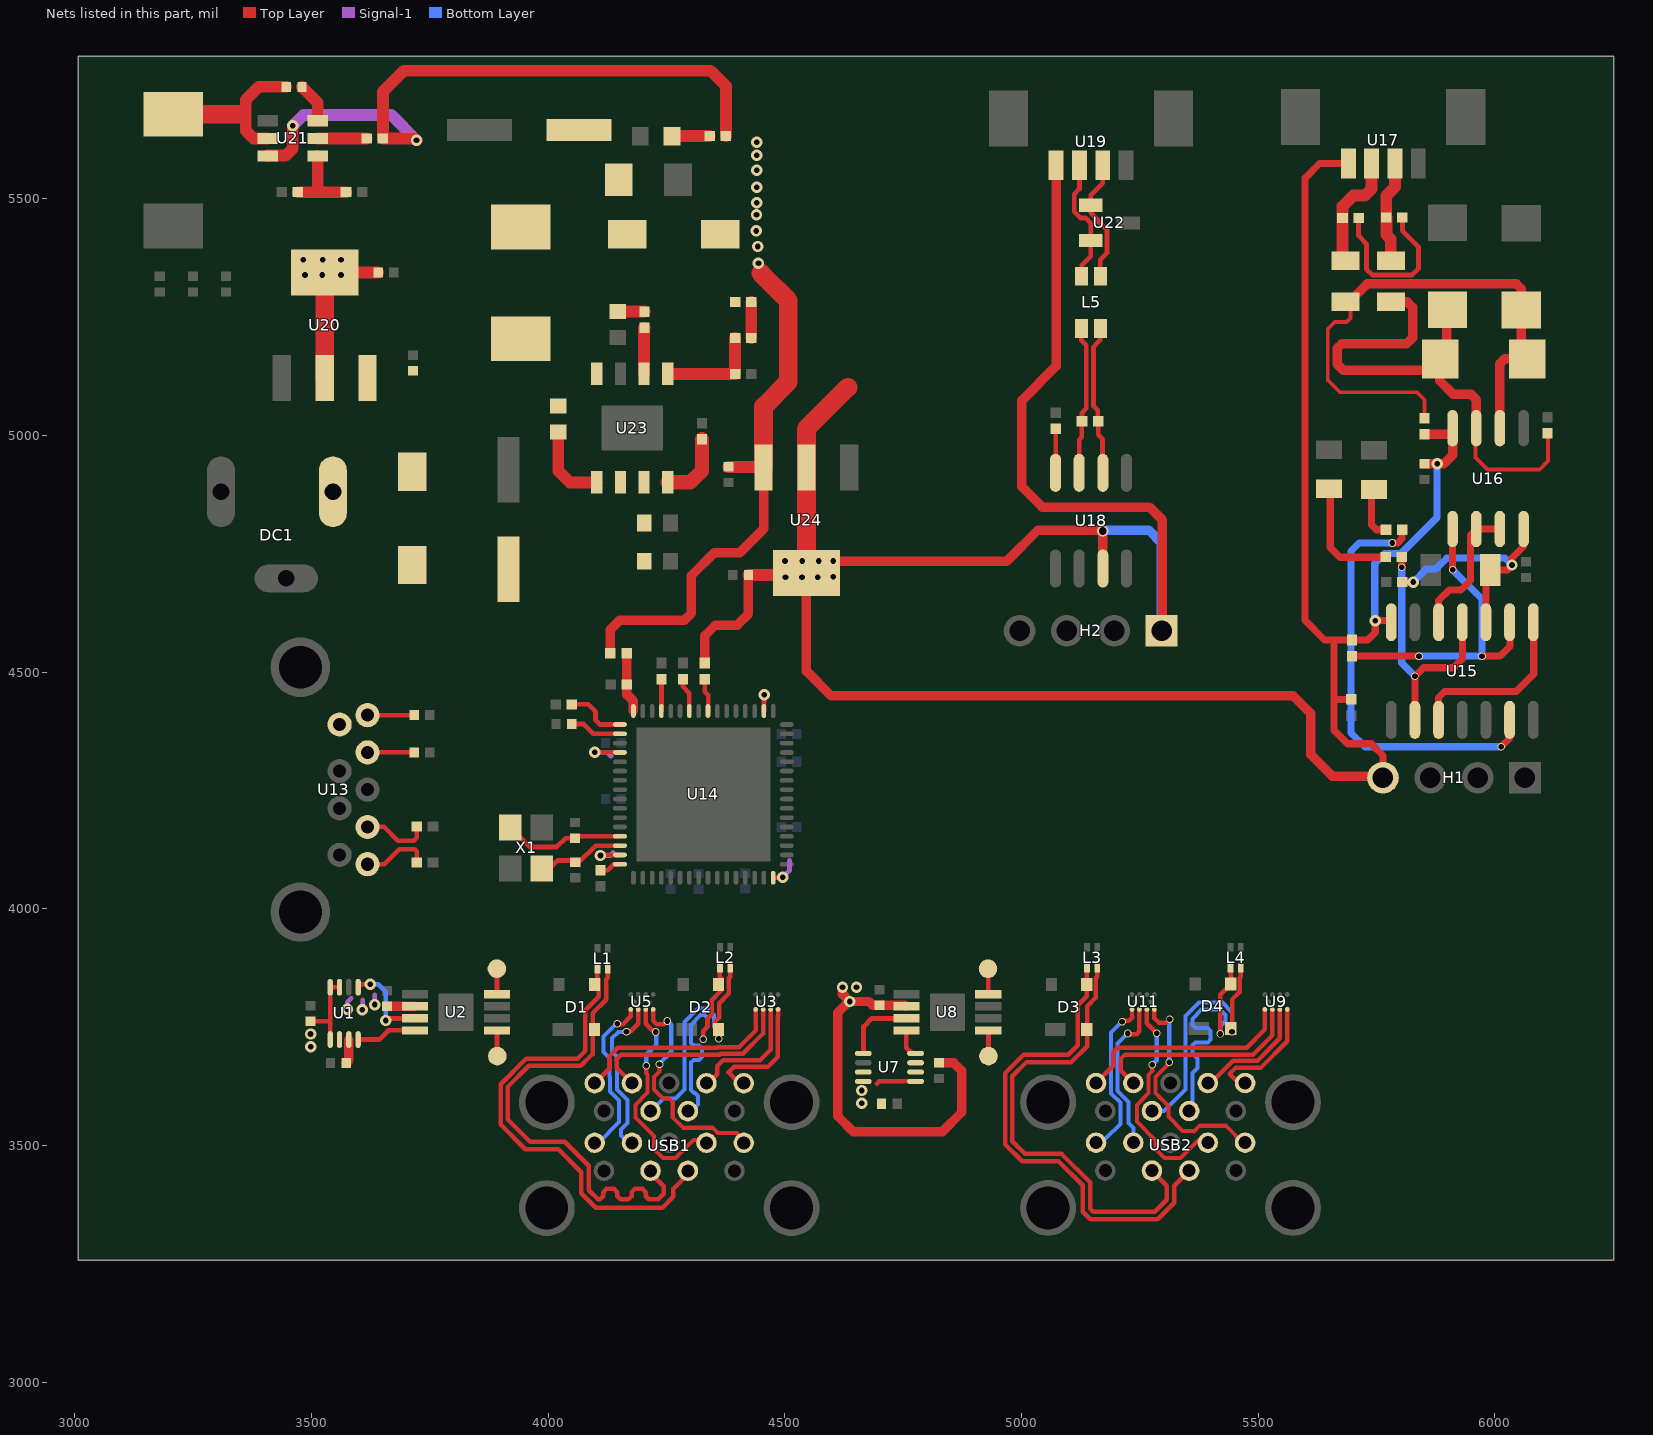
[diagram p0: the nets of this part, all layers, seen from the top]
# Altium PCB MISC51972.pcbdoc (part 2 of 3)
Units mil, origin at the board's own origin, x right, y up, seen from the top; angles counter-clockwise.
Board outline 3243 x 2543 mil, 4 copper layers (Top Layer, GND, Signal-1, Bottom Layer), stack 62.447 mil thick; 117 components, 123 nets, 473 pads, 324 vias.

## Via types
v1: diameter 24.02, hole 12, Top Layer to Bottom Layer, 276 vias
v2: diameter 16, hole 12, Top Layer to Bottom Layer, 47 vias
v3: diameter 24, hole 16, Top Layer to Bottom Layer, 1 vias

## Nets (pads, with @x,y where several pads share a name; then routed paths per layer and width w, separated by ;. In a path a pad name is that pad's centre, name@x,y a point inside that pad or via, vN(x,y) a via of type N, cw(c..) or ccw(c..) an arc to the next point about the centre after c; other vN are vias at no path point) (continued)
1.8V: C3.1 C6.1 C28.2 U1.3 U1.4 U1.5 U7.3 U7.4 U7.5 U20.2 U20.4 | length 591.4
  Top Layer w10: C3.1@3497.8,3762.76 3538.48,3762.76 3539.27,3761.97 ; U1.5@3539.27,3724.18 3539.27,3761.97 ; U1.3@3558.96,3834.62 U1.4@3539.27,3834.62 3539.27,3761.97 ; 4694.5,3631 4699.25,3635.75 U7.5@4775.99,3635.75
  Top Layer w25: U20.4@3527.7,5344.61 3640.35,5344.61 C28.2@3640.46,5344.5
  Top Layer w40: U20.2@3527.7,5121.39 U20.4@3527.7,5344.61
  other v1: 4662.5,3589.86 4662.5,3616.5 3498.5,3709 3497.8,3735.76 3485.87,5339.5 3522.76,5339.5 3562,5339.5 3482.5,5371.5 3523.5,5371.5 3561.93,5371.5
3.3V: C15.1 C36.2 H1.4 H2.1 R5.2 R6.2 R8.2 R14.2 U14.16 U14.34 U14.52 U14.63 U15.14 U16.8 U17.4 U18.3 U19.4 U24.2 U24.4 | length 7174.4
  Top Layer w10: v1@4098.5,4331.07 4151.02,4331.07 U14.52@4151.41,4330.68 ; v1@4110.15,4113.07 v1(4110.15,4112.92) 4111.38,4114.15 U14.63@4151.41,4114.15 ; U14.34@4455.54,4418.28 4455.54,4451.54 v1(4456.5,4452.5) ; U14.16@4475.23,4065.92 4494.42,4065.92 v1(4495.5,4067)
  Top Layer w15: U17.4@5690.33,5574.64 5629.64,5574.64 5599.1,5544.1 5599.1,4609.1 5640,4568.2 5659.6,4568.2 ; R5.2@5696.45,4442.7 5659.6,4442.7 ; H1.4@5763.5,4277.5 5763.5,4324.2 5738.6,4349.1 5688.6,4349.1 5659.6,4378.1 5659.6,4442.7 ; U15.14@5780.95,4605.77 5777.62,4609.1 v1(5747.1,4609.1) 5747.1,4584.1 5731.6,4568.6 5698.85,4568.6 R6.2@5698.45,4568.2 5659.6,4568.2 ; 5659.6,4442.7 5659.6,4568.2
  Top Layer w20: R14.2@4330.6,4519.64 4330.6,4577.36 4352.74,4599.5 4399,4599.5 4422.84,4623.34 C36.2@4422.84,4705.5 ; U24.4@4545.4,4709.29 4545.4,4502.6 4598,4450 5574,4450 5611,4413 5611,4326 5656.5,4280.5 5760.5,4280.5 H1.4@5763.5,4277.5 ; v1(4602.04,4735) 4969,4735 5034,4800 5170.14,4800 v3(5171.64,4798.5) U18.3@5171.64,4719.18 ; U19.4@5073.02,5571.14 5073.02,5147.02 5000.5,5074.5 5000.5,4892 5043.5,4849 5270,4849 5297.5,4821.5 5297.5,4589.71 H2.1@5295.64,4587.86 ; C15.1@5851,4940.54 v1(5878,4940.54) 5892.04,4940.54 5911.1,4959.6 5911.1,5015.01 U16.8@5910.45,5015.66 5910.45,5002.46 R8.2@5851,5002.46
  Top Layer w25: C36.2@4422.84,4705.5 4541.61,4705.5 U24.4@4545.4,4709.29
  Top Layer w40: U24.4@4545.4,4709.29 U24.2@4545.4,4932.51 4545.4,5014.4 4633,5102
  Signal-1 w10: v1(4098.5,4330.89) 4124.61,4330.89 4132.5,4323 ; v1(4110.15,4112.92) 4130.92,4112.92 4137.5,4119.5 ; v1(4495.5,4067) 4509.5,4081 4509.5,4103
  Bottom Layer w15: v1(5747.1,4609.1) 5746.1,4610.1 5746.1,4730.1 5766.6,4750.6 5801.1,4750.6 5878,4827.5 v1(5878,4940.54)
  Bottom Layer w20: v3(5171.64,4798.5) 5173.14,4800 5269,4800 5295.5,4773.5 5295.5,4588 H2.1@5295.64,4587.86
  other v1: 4501,4701 4536.05,4701 4569.5,4701 4602.04,4702.08 4500,4735 4536.48,4735 4571.39,4735
12V: C27.2 D10.1 DC1.1 U20.3
485-1: U15.12 U16.2 U16.3 | length 294.2
  Top Layer w15: U15.12@5880.95,4605.77 5880.95,4651.45 5903.6,4674.1 5928.1,4674.1 5948.1,4694.1 5948.1,4790.31 U16.2@5960.45,4802.66 U16.3@6010.45,4802.66
485-7: D6.1 D7.2 F2.1 R16.2 U16.7 | length 1151.4
  Top Layer w8: U16.7@5960.45,5015.66 5958.95,5014.16 5958.95,4953.75 5984.2,4928.5 6094.5,4928.5 6112.1,4946.1 6112.1,5003.93 R16.2@6111.45,5004.58
  Top Layer w20: F2.1@5779.95,5282.86 5814.34,5282.86 5826.1,5271.1 5826.1,5206.6 5813.5,5194 5676.5,5194 5666.6,5184.1 5666.6,5151.1 5679.1,5138.6 5861.37,5138.6 D6.1@5883.27,5160.5 ; D7.2@5899.45,5265.93 5897.95,5264.43 5897.95,5175.18 D6.1@5884.77,5162 D6.1@5883.27,5160.5 ; U16.7@5960.45,5015.66 5960.45,5076.25 5949.7,5087 5912.2,5087 5883.27,5115.93 D6.1@5883.27,5160.5
$1N3773: U1.8 U2.4 | length 128.3
  Top Layer w10: U1.8@3598.33,3724.18 3643.18,3724.18 3662.5,3743.5 3718.2,3743.5 U2.4@3718.49,3743.21
$1N3774: U1.1 U2.3 | length 192.1
  Top Layer w10: U1.1@3598.33,3834.62 3604.71,3841 v1(3624,3841) ; v1(3656.5,3764.41) 3660.89,3768.8 U2.3@3718.49,3768.8
  Bottom Layer w10: v1(3624,3841) 3641,3841 3656.5,3825.5 v1(3656.5,3764.41)
$1N3787: U7.8 U8.4 | length 60.9
  Top Layer w10: U8.4@4756.39,3743.21 4756.39,3707 4768.58,3694.81 U7.8@4775.99,3694.81
$1N3788: U7.1 U8.3 | length 154.4
  Top Layer w10: U7.1@4665.55,3694.81 4666,3695.26 4666,3751.5 4683.3,3768.8 U8.3@4756.39,3768.8
$1N3806: D1.2 L1.2 USB1.2 | length 1020.7
  Top Layer w9.5: L1.2@4125.43,3873.15 4125.43,3854.5 4122.35,3851.42 4122.35,3808.43 4093.46,3779.54 4093.46,3693.58 4068.38,3668.5 3958.51,3668.5 3914,3623.99 3914,3555.5 3961.5,3508 4034.5,3508 4085.31,3457.19 4085.31,3433.43 4085.5,3433.24 4085.5,3406 4105,3386.5 4109.17,3386.5 4115.89,3393.22 4115.89,3401.71 4122.6,3408.42 4139.17,3408.42 4145.89,3401.71 4145.89,3393.22 4152.6,3386.5 4169.17,3386.5 4175.89,3393.22 4175.89,3401.78 4182.6,3408.5 4199.17,3408.5 4205.89,3401.78 4205.89,3393.22 4212.6,3386.5 4232.35,3386.5 4244.04,3398.19 4244.04,3414.11 4217.43,3440.73 USB1.2@4217.43,3447.15
$1N3807: D1.3 L1.3 USB1.3 | length 1020.7
  Top Layer w9.5: L1.3@4103.77,3873.15 4103.77,3854.5 4106.85,3851.42 4106.85,3814.85 4077.96,3785.96 4077.96,3700 4061.96,3684 3953.5,3684 3899.5,3630 3899.5,3544.5 3951.5,3492.5 4021.5,3492.5 4070,3444 4070,3399.58 4100.58,3369 4241.32,3369 4264,3391.68 4264,3408.5 4296.17,3440.67 USB1.3@4296.17,3447.15
$1N3813: D2.3 L2.3 USB1.12 | length 496.7
  Top Layer w9.5: v2(4327.28,3724.72) 4327.28,3742.22 4335.89,3750.83 4335.89,3767.53 4345.46,3777.1 4345.46,3807.46 4365.75,3827.75 4365.75,3853.42 4362.67,3856.5 L2.3@4362.67,3875.15
  Bottom Layer w8.5: USB1.12@4294.86,3572.83 4299.03,3572.83 4307.39,3581.19 4309.83,3581.19 4315.84,3587.2 4315.84,3605.18 4309.83,3611.19 4307.39,3611.19 4301.38,3617.2 4301.38,3675.18 4307.39,3681.19 4318.48,3681.19 4324.49,3687.2 4324.49,3705.18 4318.48,3711.19 4307.39,3711.19 4301.38,3717.2 4301.38,3755.12 4321.88,3775.62 4330.38,3775.62 4336.39,3769.61 4336.39,3750.33 4327.28,3741.22 v2(4327.28,3724.72)
$1N3814: D2.2 L2.2 USB1.11 | length 537.9
  Top Layer w9.5: D2.2@4359.8,3745.56 4360,3745.36 D2.2@4360,3743 ; v2(4360,3725.5) D2.2@4360,3743 ; L2.2@4384.33,3875.15 4384.33,3856.5 4381.25,3853.42 4381.25,3821.33 4360.96,3801.04 4360.96,3770.68 4351.39,3761.11 4351.39,3751.61 D2.2@4360,3743
  Bottom Layer w8.5: USB1.11@4216.12,3572.83 4243.3,3600 4268.7,3600 4287.38,3618.68 4287.38,3761.63 4315.88,3790.12 4336.39,3790.12 4350.5,3776.01 4350.5,3751.5 4360,3742 v2(4360,3725.5)
$1N3821: D3.2 L3.2 USB2.2 | length 1001.1
  Top Layer w9.5: L3.2@5159.83,3875.15 5159.83,3856.5 5156.75,3853.42 5156.75,3812.83 5138.46,3794.54 5138.46,3710.04 5104.92,3676.5 5010.42,3676.5 4980.46,3646.54 4980.46,3509.46 5007.46,3482.46 5084.46,3482.46 5144.5,3422.42 5144.5,3367 5151.22,3360.28 5281.5,3360.28 5306.92,3385.71 5306.92,3415.53 USB2.2@5275.3,3447.15
$1N3822: D3.3 L3.3 USB2.3 | length 1049.9
  Top Layer w9.5: L3.3@5138.17,3875.15 5137.5,3874.48 5137.5,3815.5 5118.86,3796.86 5118.86,3712.36 5098.5,3692 5004,3692 4964.96,3652.96 4964.96,3503.04 5001.04,3466.96 5078.04,3466.96 5129,3416 5129,3360.58 5144.8,3344.78 5287.92,3344.78 5322.42,3379.29 5322.42,3415.53 USB2.3@5354.04,3447.15
$1N3827: D4.3 L4.3 USB2.12 | length 547.3
  Top Layer w9.5: v2(5419.76,3736) 5419.76,3819.03 5444.65,3843.92 5444.65,3853.42 5441.57,3856.5 L4.3@5441.57,3875.15
  Bottom Layer w8.5: USB2.12@5354.04,3573.13 5361,3580.09 5361,3653.56 5371.82,3664.38 5371.82,3683.56 5361,3694.38 5361,3712.36 5367.01,3718.37 5393.25,3718.37 5399.26,3724.38 5399.26,3742.36 5393.25,3748.37 5367.01,3748.37 5361,3754.38 5361,3768 5380.5,3787.5 5419.41,3787.5 5431,3775.91 5431,3763.74 5419.76,3752.5 v2(5419.76,3736)
$1N3831: D4.2 L4.2 USB2.11 | length 546.7
  Top Layer w9.5: v2(5444.5,3740.5) 5444.5,3808.8 5460.55,3824.85 5460.55,3853.81 5463.23,3856.5 L4.2@5463.23,3875.15
  Bottom Layer w8.5: USB2.11@5275.3,3573.13 5300.71,3573.13 5346.56,3618.98 5346.56,3774.07 5374.49,3802 5424.01,3802 5444.5,3781.51 v2(5444.5,3740.5)
$1N3840: U3.C1 USB1.18 | length 447.2
  Top Layer w9.5: USB1.18@4098.02,3631.89 4129.64,3663.51 4129.64,3678.35 cw(c4143.96,3680.61) 4129.5,3679.57 4128.46,3680.61 4128.46,3688.46 4147,3707 4357.02,3707 4358.31,3708.29 4403.29,3708.29 4438.26,3743.26 4438.26,3773.14 4438.13,3773.26 U3.C1@4438.13,3787.76
$1N3841: U3.C2 USB1.17 | length 447.2
  Top Layer w9.5: USB1.17@4176.76,3631.89 4145.14,3663.51 4145.14,3679.43 4143.96,3680.61 4143.96,3682.04 4153.42,3691.5 4362.03,3691.5 4364.32,3693.79 4410.71,3693.79 4453.76,3736.83 4453.76,3773.14 4453.88,3773.26 U3.C2@4453.88,3787.76
$1N3842: U3.C3 USB1.15 | length 260.1
  Top Layer w9.5: USB1.15@4334.23,3631.89 4338.39,3631.89 4357,3650.5 4357,3668.09 4369.7,3680.79 4447.71,3680.79 4469.62,3702.71 U3.C3@4469.62,3787.76
$1N3843: U3.C4 USB1.14 | length 260
  Top Layer w9.5: USB1.14@4412.98,3631.89 4403.61,3631.89 4380.61,3654.89 4392.01,3666.29 4463.46,3666.29 4485.24,3688.08 4485.24,3773.14 4485.37,3773.26 U3.C4@4485.37,3787.76
$1N3853: U9.C1 USB2.18 | length 463
  Top Layer w9.5: USB2.18@5157.19,3632.19 5193.46,3668.46 5193.46,3697.46 5203,3707 5475.49,3707 5514.08,3745.59 U9.C1@5514.08,3787.76
$1N3854: U9.C2 USB2.17 | length 458.4
  Top Layer w9.5: USB2.17@5235.93,3632.19 5208.96,3659.16 5208.96,3683 5218.46,3692.5 5489.5,3692.5 5529.7,3732.7 5529.7,3773.14 5529.83,3773.26 U9.C2@5529.83,3787.76
$1N3855: U9.C3 USB2.15 | length 252.4
  Top Layer w9.5: USB2.15@5393.41,3632.19 5399.46,3632.19 5446.77,3679.5 5498.19,3679.5 5545.69,3727 5545.69,3773.14 5545.57,3773.26 U9.C3@5545.57,3787.76
$1N3856: U9.C4 USB2.14 | length 258.4
  Top Layer w9.5: USB2.14@5472.15,3632.19 5458.81,3632.19 5439.39,3651.61 5452.78,3665 5505.62,3665 5561.19,3720.58 5561.19,3773.14 5561.32,3773.26 U9.C4@5561.32,3787.76
$1N3865: U5.C4 USB1.5 | length 481.2
  Top Layer w8.5: v2(4235,3672) 4235,3656.49 4223.61,3645.1 4223.61,3618.68 4242.29,3600 4255.5,3600 4262.98,3592.52 4262.98,3559.62 4284.81,3537.79 4347.44,3537.79 4358.82,3526.41 4398.47,3526.41 4412.98,3511.91 USB1.5@4412.98,3505.9
  Top Layer w9.5: U5.C4@4221.62,3787.76 4221.62,3773.26 4221.49,3773.14 4221.49,3763.64 4228.21,3756.92 4245,3756.92 v2@4251.34,3763.26
  Bottom Layer w9.5: v2(4235,3672) 4235,3673.5 4259.5,3698 4259.5,3755.2 v2(4251.34,3763.36)
$1N3866: U5.C3 USB1.6 | length 480.7
  Top Layer w8.5: v2(4207,3669) 4207,3652.5 4210.11,3649.39 4210.11,3611.91 4184.24,3586.04 4184.24,3559.62 4223.61,3520.25 4223.61,3492.69 4242.29,3474.01 4268.7,3474.01 4306.6,3511.91 4328.23,3511.91 USB1.6@4334.23,3505.9
  Top Layer w9.5: U5.C3@4205.87,3787.76 4205.87,3773.26 4205.99,3773.14 4205.99,3757.22 4221.79,3741.42 4225.96,3741.42 v2(4227.34,3740.04)
  Bottom Layer w9.5: v2(4207,3669) 4207,3692 4228.5,3713.5 4228.5,3738.88 v2(4227.34,3740.04)
$1N3867: U5.C2 USB1.8 | length 352.3
  Top Layer w9.5: v2(4165.28,3740.55) 4173.05,3740.55 4190.01,3757.51 4190.01,3773.5 4190.13,3773.62 U5.C2@4190.13,3787.76
  Bottom Layer w8.5: v2(4165.28,3740.55) 4148.05,3740.55 4134.99,3727.49 4134.99,3698.4 4144.87,3688.52 4144.87,3618.68 4167,3596.55 4167,3548 4153.5,3534.5 4153.5,3521.5 4169.1,3505.9 USB1.8@4176.76,3505.9
$1N3868: U5.C1 USB1.9 | length 354.9
  Top Layer w9.5: v2(4146.02,3757.35) 4147.65,3757.35 4148.25,3756.75 4157.75,3756.75 4174.51,3773.5 4174.38,3773.62 U5.C1@4174.38,3787.76
  Bottom Layer w8.5: USB1.9@4098.02,3505.9 4105.81,3505.9 4149.58,3549.68 4149.58,3594.92 4129.9,3614.6 4129.9,3645.1 4129,3646 4129,3685.3 4116.5,3697.8 4116.5,3730.5 4143.35,3757.35 v2(4146.02,3757.35)
$1N3877: U11.C4 USB2.5 | length 482
  Top Layer w8.5: 5282.55,3618.74 5282.79,3618.5 ; v2(5312.12,3675.85) 5312.12,3674.74 5282.79,3645.4 5282.79,3618.5 ; USB2.5@5472.15,3506.2 5467.16,3506.2 5431.36,3542 5376.11,3542 5364.1,3529.99 5362.86,3531.24 5339.84,3531.24 5310,3561.08 5310,3584.1 5282.79,3611.31 5282.79,3618.5
  Top Layer w9.5: U11.C4@5280.47,3787.76 5280.47,3769.53 5290.25,3759.75 5305.5,3759.75 v2(5312.62,3766.88)
  Bottom Layer w9.5: v2(5312.12,3675.85) 5312.12,3766.38 v2(5312.62,3766.88)
$1N3878: U11.C3 USB2.6 | length 473.7
  Top Layer w8.5: v2(5276,3670.85) 5276,3657.7 5267.82,3649.52 5267.82,3610.74 5243.42,3586.34 5243.42,3550.58 5282.79,3511.21 5282.79,3492.99 5301.47,3474.31 5336.11,3474.31 5374.01,3512.21 5387.4,3512.21 USB2.6@5393.41,3506.2
  Top Layer w9.5: U11.C3@5264.72,3787.76 5264.72,3758.28 v2(5285.5,3737.5)
  Bottom Layer w9.5: v2(5276,3670.85) 5285.5,3680.35 v2(5285.5,3737.5)
$1N3879: U11.C2 USB2.8 | length 327.7
  Top Layer w9.5: v2(5224.41,3736.82) 5225.74,3735.5 5243,3735.5 5248.85,3741.36 5248.85,3773.14 5248.98,3773.26 U11.C2@5248.98,3787.76
  Bottom Layer w8.5: v2(5224.41,3736.82) 5223.82,3736.82 5202.58,3715.58 5202.58,3615.92 5226,3592.51 5226,3547.5 5235.93,3537.57 USB2.8@5235.93,3506.2
$1N3880: U11.C1 USB2.9 | length 343.8
  Top Layer w9.5: v2(5212.28,3761.81) 5214.11,3763.64 5226.64,3763.64 5233.35,3770.35 5233.35,3773.14 5233.23,3773.26 U11.C1@5233.23,3787.76
  Bottom Layer w8.5: USB2.9@5157.19,3506.2 5165.69,3514.7 5177.71,3514.7 5208.76,3545.75 5208.76,3590.65 5189.08,3610.33 5189.08,3738.61 v2(5212.28,3761.81)
$1N5034: C9.2 U14.62 X1.1 | length 187.8
  Top Layer w10: X1.1@3986.47,4085.89 4003.39,4085.89 4020,4102.5 4053.34,4102.5 C9.2@4057,4098.84 4064.84,4098.84 4099.83,4133.83 U14.62@4151.41,4133.83
$1N5035: C10.2 U14.61 X1.3 | length 258.4
  Top Layer w10: X1.3@3919.53,4172.51 3961.05,4131 4018,4131 4036.56,4149.56 C10.2@4056.7,4149.56 4060.66,4153.52 U14.61@4151.41,4153.52
$1N5041: R3.1 U14.64 | length 46.6
  Top Layer w10: R3.1@4110,4082.04 4125.54,4082.04 4137.96,4094.46 U14.64@4151.41,4094.46
$1N5046: C17.1 U14.50 | length 110.6
  Top Layer w10: C17.1@4049.34,4390.72 4074.78,4390.72 4095.45,4370.05 U14.50@4151.41,4370.05
$1N5048: R11.1 U14.49 | length 129.5
  Top Layer w10: R11.1@4049.84,4432.4 4084.1,4432.4 4100,4416.5 4100,4399 4109.26,4389.74 U14.49@4151.41,4389.74
$1N5050: R7.1 R9.1 U14.48 | length 128.1
  Top Layer w20: R7.1@4165.33,4540.28 4165.33,4474.77 R9.1@4166.2,4473.9 4166.2,4452.8 4179.95,4439.05 U14.48@4179.95,4418.28
$1N5101: R12.1 U14.45 | length 67.3
  Top Layer w10: U14.45@4239.01,4418.28 4239.1,4418.37 R12.1@4239.1,4485.56
$1N5103: R13.1 U14.42 | length 72.7
  Top Layer w10: R13.1@4284.8,4485.56 4284.8,4469.2 4298,4456 U14.42@4298,4418.34
$1N5105: R14.1 U14.40 | length 70.6
  Top Layer w10: R14.1@4330.6,4485.56 4330.6,4458.9 4338,4451.5 4338,4418.85 U14.40@4337.43,4418.28
$1N8075: R6.1 U15.9 U16.1 | length 687.8
  Top Layer w15: R6.1@5698.45,4534.12 v2(5839.6,4534.1) ; U16.1@5910.45,4802.66 5910.6,4802.51 v2(5910.6,4716.6) ; v2(5972.6,4534.1) 6011.1,4534.1 6032.1,4555.1 6032.1,4604.62 U15.9@6030.95,4605.77
  Bottom Layer w15: v2(5839.6,4534.1) v2(5972.6,4534.1) 5972.6,4654.6 v2(5910.6,4716.6)
$1N8076: R17.1 U15.2 U15.11 | length 548.7
  Top Layer w15: v2(5803.1,4722.1) 5803.1,4742.77 R17.1@5803.49,4743.16 ; U15.2@5830.95,4399.55 v2(5830.95,4491.6) 5848.95,4509.6 5912.6,4509.6 5931.6,4528.6 5931.6,4605.12 U15.11@5930.95,4605.77
  Bottom Layer w15: v2(5803.1,4722.1) 5803.1,4519.45 v2(5830.95,4491.6)
$1N8077: R18.2 U15.6 | length 915
  Top Layer w15: v2(5783.1,4773.1) 5794.6,4773.1 5803.95,4782.45 R18.2@5803.95,4801.16 ; v2(6013.1,4342.6) 6030.95,4360.45 U15.6@6030.95,4399.55
  Bottom Layer w15: v2(5783.1,4773.1) 5713.1,4773.1 5696.1,4756.1 5696.1,4372.1 5725.6,4342.6 v2(6013.1,4342.6)
$1N8081: U15.3 U15.8 | length 378.8
  Top Layer w15: U15.3@5880.95,4399.55 5880.95,4446.45 5893.6,4459.1 6045.1,4459.1 6082.1,4496.1 6082.1,4604.62 U15.8@6080.95,4605.77
$1N8120: R4.2 R10.2 | length 358
  Top Layer w10: R4.2@5711.99,5460.16 5711.99,5422.01 5728.5,5405.5 5728.5,5352 5741,5339.5 5825,5339.5 5838.5,5353 5838.5,5399 5804.49,5433.01 R10.2@5804.49,5461.16
$1N8121: F2.2 R10.1 U17.2 | length 216.7
  Top Layer w25: F2.2@5779.95,5369.47 5779.95,5415.25 5770.6,5424.6 5770.6,5460.97 R10.1@5770.41,5461.16 5770.41,5506.91 5788.76,5525.26 U17.2@5788.76,5574.64
$1N8129: D5.1 D6.2 F1.1 R8.1 U16.6 | length 1189.9
  Top Layer w8: F1.1@5684.45,5282.86 5694.6,5272.71 5694.6,5248.1 5686.6,5240.1 5661.6,5240.1 5646.6,5225.1 5646.6,5117.6 5672.6,5091.6 5835.1,5091.6 5851,5075.7 R8.1@5851,5036.54
  Top Layer w20: F1.1@5684.45,5282.86 5692.36,5282.86 5730.5,5321 6044.7,5321 6055.45,5310.25 D5.1@6055.45,5265.43 6055.45,5162 6020.5,5162 6010.45,5151.95 U16.6@6010.45,5015.66
$1N8138: R17.2 TXD1.1 | length 251.1
  Top Layer w15: TXD1.1@5649.45,4887.82 5652.1,4885.17 5652.1,4763.6 5672.54,4743.16 R17.2@5769.41,4743.16
$1N8140: R18.1 RXD1.1 | length 112
  Top Layer w15: RXD1.1@5744.45,4886.32 5739.1,4880.97 5739.1,4811.6 5749.54,4801.16 R18.1@5769.87,4801.16
$1N8159: L5.4 R22.2 U18.7 | length 315.6
  Top Layer w10: U18.7@5121.64,4921.54 5121.64,4991.14 5127,4996.5 5127,5029.75 R22.2@5127.6,5030.36 5127.6,5048.6 5136.5,5057.5 5136.5,5190.5 5126,5201 5126,5225.28 L5.4@5126.96,5226.24
$1N8164: L5.1 R22.1 U18.6 | length 318.8
  Top Layer w10: L5.1@5166.33,5226.24 5166.33,5202.33 5152,5188 5152,5062.5 5161,5053.5 5161,5031.04 R22.1@5161.68,5030.36 5161.68,5001.82 5171,4992.5 5171,4922.18 U18.6@5171.64,4921.54
$1N8180: R19.1 U18.8 | length 93
  Top Layer w10: U18.8@5071.64,4921.54 5071.64,4950.54 5072.14,4951.04 R19.1@5072.14,5014.36
$1N8697: C7.1 U13.9 | length 98.7
  Top Layer w9.5: U13.9@3618.12,4409.47 3618.34,4409.68 C7.1@3716.71,4409.68
$1N8703: C8.1 U13.8 | length 98.5
  Top Layer w9.5: U13.8@3618.18,4330.78 C8.1@3716.71,4330.78
$1N8823: R1.1 U13.6 | length 142.8
  Top Layer w9.5: U13.6@3618.12,4173.25 3653.21,4173.24 3682.32,4144.13 3715.7,4144.13 3722.41,4150.85 R1.1@3722.41,4174.48
$1N8893: R2.1 U13.5 | length 142.8
  Top Layer w9.5: U13.5@3618.12,4094.51 3653.21,4094.5 3684.83,4126.12 3718.21,4126.12 3722.41,4121.92 R2.1@3722.41,4098.28
$1N10185: R24.2 R26.1 | length 76.2
  Top Layer w25: R26.1@4428.74,5206.35 R24.2@4428.74,5282.6
$1N10186: C30.2 C31.1 D9.1 L7.2
$1N10189: LED1.1 R25.2 | length 79.7
  Top Layer w25: LED1.1@4261.47,5632.7 R25.2@4341.16,5632.7
$1N10190: C37.1 R29.2 | length 56
  Top Layer w25: C37.1@4147.02,5262.04 R29.2@4203,5262.04
$1N10191: C29.2 U23.1 | length 173.7
  Top Layer w25: C29.2@4021.1,5007.6 4021.1,4925.4 4045.5,4901 4101.9,4901 U23.1@4102.3,4901.4
$1N10192: C32.1 C33.2 C34.2 D10.2 U23.2 U23.3
$1N10193: R27.2 U23.4 | length 148.7
  Top Layer w30: U23.4@4252.3,4901.4 4299.9,4901.4 4324.5,4926 R27.2@4324.5,4992.32
$1N10194: C29.1 L7.1 U23.8
$1N10195: R29.1 U23.6 | length 97.8
  Top Layer w25: U23.6@4202.3,5130.4 4202.3,5227.26 R29.1@4203,5227.96
$1N10197: R26.2 R28.1 U23.5 | length 218.7
  Top Layer w25: U23.5@4252.3,5130.4 4394.36,5130.4 R28.1@4394.66,5130.1 R26.2@4394.66,5206.35
$1N10661: C22.1 L6.2 U21.2 | length 358.4
  Top Layer w25: U21.2@3406.85,5628 3377,5628 3361,5644 3361,5709.5 3388.5,5737 C22.1@3446.46,5737
  Top Layer w40: L6.2@3207.9,5678.91 3351.43,5678.91
$1N10662: C22.2 U21.6 | length 85.5
  Top Layer w25: C22.2@3479.54,5737 3513.15,5703.39 U21.6@3513.15,5665.4
$1N10665: R20.1 U21.5 | length 103.5
  Top Layer w25: U21.5@3513.15,5628 3513.25,5627.9 R20.1@3616.56,5627.9
$1N10667: R21.1 R23.1 U21.4 | length 178
  Top Layer w25: R21.1@3470.94,5514.3 3513.19,5514.3 R23.1@3572.66,5514.3 ; 3513.15,5514.34 U21.4@3513.15,5590.6
$1N18293: U8.8 U10.1 | length 54.1
  Top Layer w10: U10.1@4929,3873.8 4929.61,3873.19 U8.8@4929.61,3819.99
$1N18297: U8.5 U12.1 | length 54.3
  Top Layer w10: U8.5@4929.61,3743.21 4930,3742.82 U12.1@4930,3689.1
$1N18319: U2.8 U4.1 | length 53.9
  Top Layer w10: U4.1@3891.5,3873.8 3891.71,3873.59 U2.8@3891.71,3819.99
$1N18323: U2.5 U6.1 | length 54.4
  Top Layer w10: U2.5@3891.71,3743.21 3891.71,3689.69 U6.1@3892.3,3689.1
$1N24710: L5.3 U19.3 U22.2 | length 268.2
  Top Layer w10: U19.3@5122.24,5571.14 5122.24,5521.24 5111,5510 5111,5473.34 5124.34,5460 5135,5460 5146.27,5448.73 U22.2@5146.27,5411.96 5146.27,5379.27 5126.96,5359.96 L5.3@5126.96,5336.48
$1N24718: L5.2 U19.2 U22.1 | length 265.1
  Top Layer w10: L5.2@5166.33,5336.48 5166.33,5371.83 5180.5,5386 5180.5,5433.5 5161.77,5452.23 5161.77,5455.15 5146.27,5470.65 U22.1@5146.27,5486.76 5146.27,5508.27 5171.45,5533.45 U19.2@5171.45,5571.14
$1N31164: F1.2 R4.1 U17.3 | length 247.6
  Top Layer w25: F1.2@5684.45,5369.47 5678.1,5375.82 5678.1,5484.6 5700.6,5507.1 5725.1,5507.1 5739.55,5521.55 U17.3@5739.55,5574.64
D1-: D8.1 R15.1 U15.10 U16.4 | length 511.8
  Top Layer w15: R15.1@5804.53,4691.16 5827.04,4691.16 v1(5827.6,4690.6) ; U15.10@5980.95,4605.77 5980.95,4706.67 D8.1@5990.44,4716.16 6026.16,4716.16 6035.1,4725.1 v1@6035.1,4727.6 ; v1(6036.1,4726.6) v1@6035.1,4727.6 ; U16.4@6060.45,4802.66 6060.45,4765.45 6035.1,4740.1 v1@6035.1,4727.6
  Bottom Layer w15: v1(5827.6,4690.6) 5855.6,4718.6 5875.6,4718.6 5897.6,4740.6 5897.6,4741.6 ; 5897.67,4741.67 6021.03,4741.67 v1(6036.1,4726.6)
D5.0V: C1.2 C2.1 C4.2 C5.1 C35.2 D9.2 R7.2 R20.2 R24.1 R25.1 U1.6 U1.7 U2.2 U7.6 U7.7 U8.2 U13.1 U21.3 U24.3 | length 3634
  Top Layer w20: C1.2@3573.04,3674.3 3578.64,3679.9 U1.7@3578.64,3724.18 ; C2.1@3659.5,3794.46 U2.2@3718.43,3794.46 ; R7.2@4131.25,4540.28 4131.25,4590.25 4150.5,4609.5 4287,4609.5 4302,4624.5 4302,4704 4351,4753 4405,4753 4454.85,4802.85 U24.3@4454.85,4932.51 ; v1(4621.5,3834.5) 4621.5,3820.04 v1(4637.04,3804.5) ; U8.2@4756.39,3794.4 4754.33,3796.46 C5.1@4699.5,3796.46 4685.54,3796.46 4677.5,3804.5 v1(4637.04,3804.5) ; C4.2@4825.5,3675.04 4856.46,3675.04 4873.5,3658 4873.5,3570.5 4832,3529 4644.5,3529 4611.5,3562 4611.5,3781 4635,3804.5 v1(4637.04,3804.5)
  Top Layer w25: U21.3@3406.85,5590.6 3406.85,5591.35 3407,5591.5 3445,5591.5 3460,5606.5 v1(3460,5654.5) ; v1(3721.5,5624) 3717.6,5627.9 R20.2@3650.64,5627.9 3650.5,5628.04 3650.5,5726.5 3695,5771 4343,5771 4375.24,5738.76 R25.1@4375.24,5632.7 ; C35.2@4380.5,4934.04 4453.32,4934.04 U24.3@4454.85,4932.51
  Top Layer w40: 4449,5343.5 4507,5285.5 4507,5113.5 4454.85,5061.35 U24.3@4454.85,4932.51
  Signal-1 w10: v1(3575.5,3788) 3575.5,3803 3584,3811.5 ; v1(3607.27,3787.18) 3608,3787.91 3608,3807.5 ; v1(3633.5,3798) 3633.5,3819
  Signal-1 w25: v1(3460,5654.5) 3483,5677.5 3668,5677.5 v1(3721.5,5624)
  other v1: 4651.3,3834.5 4444,5364 4442.5,5399.5 4439.5,5432.5 4440,5466.95 4440.5,5491.92 4440.5,5525 4440.5,5560.6 4440.5,5592.1 4440.5,5620